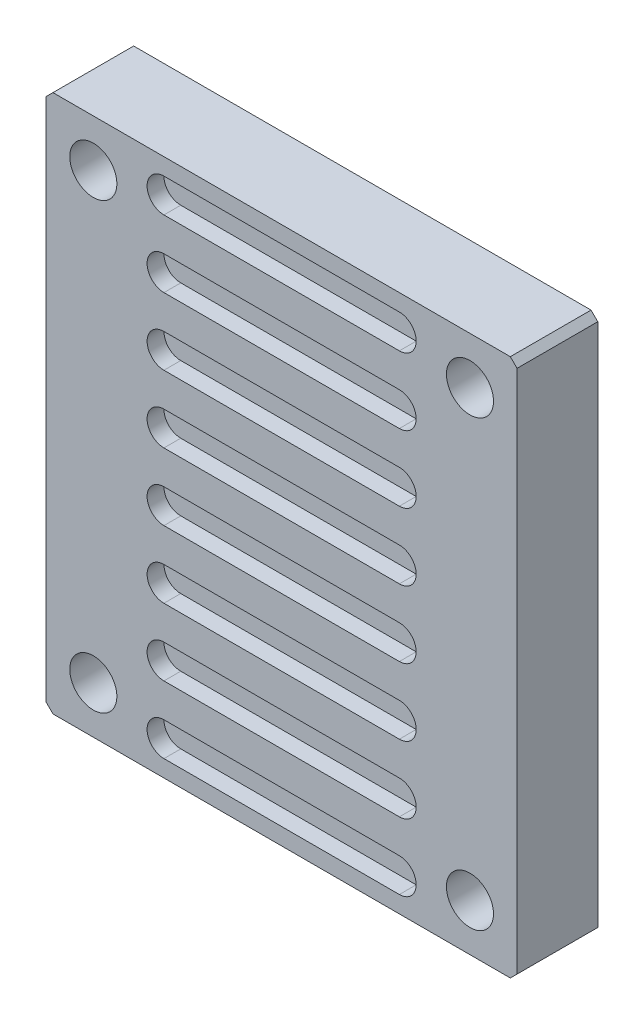
SolidWorks part; units mm, degrees
ref_plane "前视" through (0, 0, 0) normal (0, 0, 1) x (1, 0, 0)
ref_plane "上视" through (0, 0, 0) normal (0, 1, 0) x (1, 0, 0)
ref_plane "右视" through (0, 0, 0) normal (1, 0, 0) x (0, 0, -1)
sketch "草图1" plane through (0, 0, 0) normal (0, 0, 1) x (1, 0, 0)
  line L1 (0, 0) -> (70, 0)
  line L2 (0, 0) -> (0, -80)
  line L3 (0, -80) -> (70, -80)
  line L4 (70, 0) -> (70, -80)
  dimension "D1" = 70
  dimension "D2" = 80
extrude "凸台-拉伸1" add sketch "草图1" along normal blind 12
chamfer "倒角1" distance 1 angle 45 4 edges at (0, -80, 6) (70, -80, 6) (70, 0, 6) (0, 0, 6)
sketch "草图2" plane through (0, 0, 12) normal (0, 0, 1) x (1, 0, 0)
  line L0 (17.5, -5) -> (52.5, -5) construction
  line L1 (17.5, -2.5) -> (52.5, -2.5)
  line L2 (17.5, -7.5) -> (52.5, -7.5)
  line L3 (35, -2.5) -> (35, 0) construction
  line L4 (69, 0) -> (1, 0) construction
  arc A0 (17.5, -2.5) -> (17.5, -7.5) centre (17.5, -5) ccw
  arc A1 (52.5, -7.5) -> (52.5, -2.5) centre (52.5, -5) ccw
  point P2 (35, -5)
  dimension "D1" = 5
  dimension "D2" = 2.5
  dimension "D3" = 35
extrude "切除-拉伸1" cut sketch "草图2" against normal blind 2.5
pattern_linear "阵列(线性)1" count 8 spacing 10 along (0, -1, 0) of "切除-拉伸1"
hole_wizard "Ø7.0 (7) 直径孔1" positions "草图4" profile "草图3" hole size "Ø7.0" standard "ISO" end condition through all
sketch "草图4" plane through (0, 0, 0) normal (0, 0, -1) x (-1, 0, 0)
  line L1 (-7, -73) -> (-63, -73)
  line L2 (-7, -73) -> (-7, -7)
  line L3 (-7, -7) -> (-63, -7)
  line L4 (-63, -73) -> (-63, -7)
  line L5 (-35, -73) -> (-35, -80) construction
  line L6 (-1, -80) -> (-69, -80) construction
  line L8 (-63, -40) -> (-70, -40) construction
  line L9 (-70, -79) -> (-70, -1) construction
  point P0 (-7, -73)
  point P2 (-7, -7)
  point P4 (-63, -73)
  point P6 (-63, -7)
  dimension "D1" = 7
  dimension "D2" = 7
sketch "草图3" plane through (7, -73, 0) normal (1, 0, 0) x (0, 1, 0)
  line L0 (0, 0) -> (0, 12)
  line L1 (0, 12) -> (3.5, 12)
  line L2 (3.5, 12) -> (3.5, 0)
  line L5 (3.5, 0) -> (0, 0)
  line L11 (0, -6.35) -> (0, 107.95) construction
  dimension "通孔孔直径" = 7
  dimension "通孔孔深度" = 12
